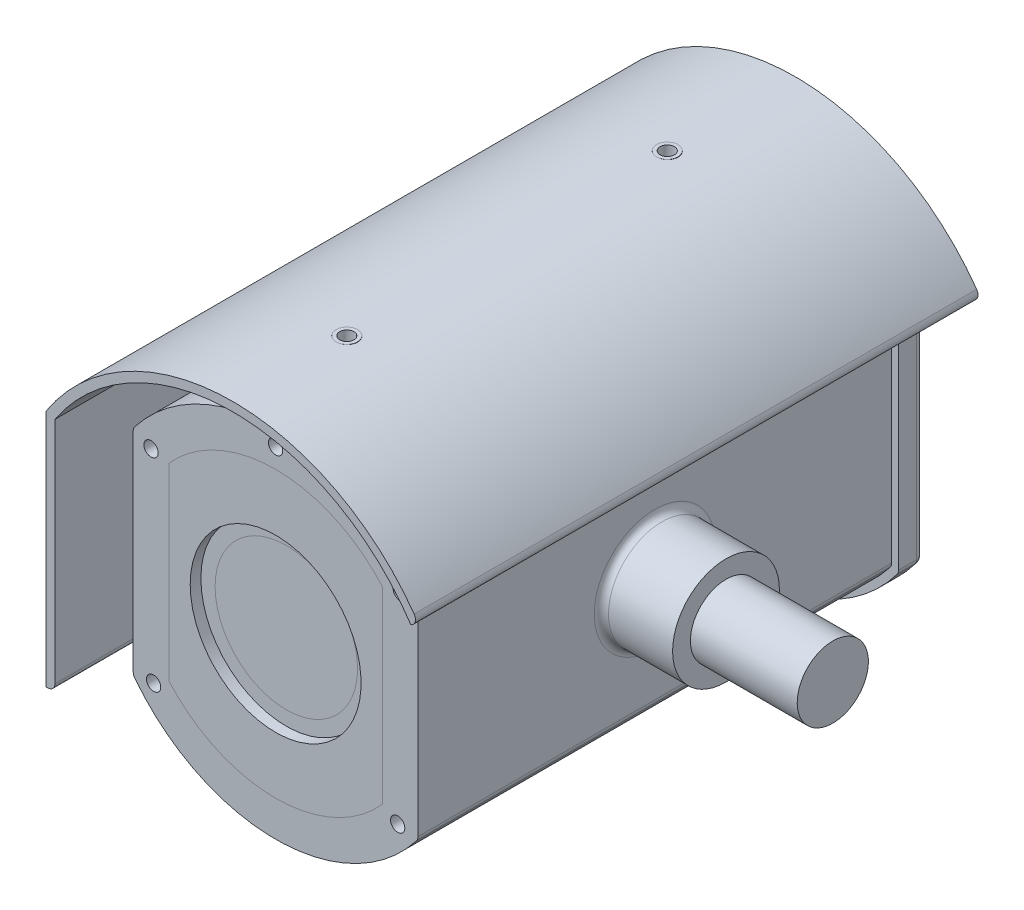
from build123d import *

# Parameters (mm, degrees)
BOSS_EXTRUDE1_DEPTH      = 140
CUT_EXTRUDE1_DEPTH       = 7
BOSS_EXTRUDE2_DEPTH      = 12
BOSS_EXTRUDE2_DEPTH_BACK = 146
SKETCH4_R                = 24
SKETCH4_R_2              = 20
BOSS_EXTRUDE3_DEPTH      = 4
CUT_EXTRUDE2_START       = -7
SKETCH5_R                = 20
CUT_EXTRUDE2_DEPTH       = 7
SKETCH6_R                = 11
CUT_EXTRUDE3_DEPTH       = 1
DOME1_FACE_RADIUS        = 11
DOME1_HEIGHT             = 5
SKETCH7_R                = 3
BOSS_EXTRUDE4_DEPTH      = 12.5
SKETCH8_R                = 2
CUT_EXTRUDE4_DEPTH       = 17
BOSS_EXTRUDE5_REACH      = 198.256
BOSS_EXTRUDE5_END_RADIUS = 50
SKETCH9_R                = 3
SKETCH10_R               = 2
CUT_EXTRUDE5_DEPTH       = 17
BOSS_EXTRUDE6_DEPTH      = 7
SKETCH12_W               = 70
SKETCH12_H               = 3.5
CUT_EXTRUDE6_DEPTH       = 5
SKETCH14_R               = 20
BOSS_EXTRUDE7_DEPTH      = 2
SKETCH15_R               = 24
BOSS_EXTRUDE8_DEPTH      = 5
SKETCH16_R               = 2
CUT_EXTRUDE8_DEPTH       = 5
CUT_EXTRUDE7_DEPTH       = 303.977741111
CUT_EXTRUDE7_DEPTH_BACK  = 303.977741111
SKETCH13_R               = 124.287084565
SKETCH17_R               = 10
BOSS_EXTRUDE9_DEPTH      = 50
SKETCH18_R               = 15
SKETCH18_R_2             = 10
BOSS_EXTRUDE10_DEPTH     = 20
FILLET1_R                = 2
SCALE1_SCALE             = 0.5


with BuildPart() as part:
    # Sketch1 → Boss-Extrude1 (new body)
    with BuildSketch(Plane.XY):
        with BuildLine():
            Line((-40, -30), (-40, 30))
            ThreePointArc((-40, 30), (0, 50), (40, 30))
            Line((40, 30), (40, -30))
            ThreePointArc((40, -30), (0, -50), (-40, -30))
        make_face()
    extrude(amount=BOSS_EXTRUDE1_DEPTH)

    # Sketch2 → Cut-Extrude1 (cut)
    with BuildSketch(Plane.XY.offset(140)):
        with BuildLine():
            Line((-30, 26.457513111), (-30, -26.457513111))
            ThreePointArc((-30, -26.457513111), (0, -40), (30, -26.457513111))
            Line((30, -26.457513111), (30, 26.457513111))
            ThreePointArc((30, 26.457513111), (0, 40), (-30, 26.457513111))
        make_face()
    extrude(amount=-CUT_EXTRUDE1_DEPTH, mode=Mode.SUBTRACT)

    # Sketch4 → Boss-Extrude3 (add)
    with BuildSketch(Plane.XY.offset(133)):
        Circle(SKETCH4_R)
        Circle(SKETCH4_R_2, mode=Mode.SUBTRACT)
    extrude(amount=BOSS_EXTRUDE3_DEPTH)

    # Sketch5 → Cut-Extrude2 (cut)
    with BuildSketch(Plane.XY.offset(133).offset(CUT_EXTRUDE2_START)):
        Circle(SKETCH5_R)
    extrude(amount=CUT_EXTRUDE2_DEPTH, mode=Mode.SUBTRACT)

    # Sketch6 → Cut-Extrude3 (cut)
    with BuildSketch(Plane.XY.offset(126)):
        Circle(SKETCH6_R)
    extrude(amount=-CUT_EXTRUDE3_DEPTH, mode=Mode.SUBTRACT)

    # Dome1: a dome of height H over a round flat face of radius A is a cap of a sphere of radius (A * A + H * H) / (2 * H)
    dome1_r = (DOME1_FACE_RADIUS * DOME1_FACE_RADIUS + DOME1_HEIGHT * DOME1_HEIGHT) / (2 * DOME1_HEIGHT)
    dome1_base = Plane((0, 0, 125), z_dir=(0, 0, 1))
    with Locations(dome1_base.offset(DOME1_HEIGHT - dome1_r)):
        dome1_ball = Sphere(dome1_r, mode=Mode.PRIVATE)
    add(split(dome1_ball, bisect_by=dome1_base, keep=Keep.TOP, mode=Mode.PRIVATE))



with BuildPart() as body_2:
    # Sketch3 → Boss-Extrude2 (new, two sides: drawn at the far end of the back side and taken through both)
    with BuildSketch(Plane.XY.offset(140).offset(-BOSS_EXTRUDE2_DEPTH_BACK)):
        with BuildLine():
            Line((52.5, -33.166247904), (52.5, 33.911649916))
            ThreePointArc((52.5, 33.911649916), (0.380386371, 62.498842439), (-52.083333333, 34.5481749))
            Line((-52.083333333, 34.5481749), (-50, 33.166247904))
            ThreePointArc((-50, 33.166247904), (0, 60), (50, 33.166247904))
            Line((50, 33.166247904), (50, -33.166247904))
            Line((50, -33.166247904), (52.5, -33.166247904))
        make_face()
    extrude(amount=BOSS_EXTRUDE2_DEPTH + BOSS_EXTRUDE2_DEPTH_BACK)


with BuildPart() as part_1:
    add(part.part)

    add(body_2.part)  # Boss-Extrude4 merges body 2
    # Sketch7 → Boss-Extrude4 (add)
    with BuildSketch(Plane(origin=(52.5, 0, 0), x_dir=(0, 0, -1), z_dir=(1, 0, 0))):
        with Locations(Location((-120, 0, 0), (0, 0, 270))):
            Circle(SKETCH7_R)
        with Locations(Location((-30, 0, 0), (0, 0, 270))):
            Circle(SKETCH7_R)
    extrude(amount=-BOSS_EXTRUDE4_DEPTH)

    # Sketch8 → Cut-Extrude4 (cut)
    with BuildSketch(Plane(origin=(52.5, 0, 0), x_dir=(0, 0, -1), z_dir=(1, 0, 0))):
        with Locations((-120, 0)):
            Circle(SKETCH8_R)
        with Locations((-30, 0)):
            Circle(SKETCH8_R)
    extrude(amount=-CUT_EXTRUDE4_DEPTH, mode=Mode.SUBTRACT)

    # Boss-Extrude5: up to this cylinder (the profile starts outside it)
    boss_extrude5_end = Plane(origin=(0, 0, 75), z_dir=(0, 0, -1)) * Cylinder(BOSS_EXTRUDE5_END_RADIUS, 587.512, mode=Mode.PRIVATE)
    # Sketch9 → Boss-Extrude5 (add, up to the surface)
    with BuildSketch(Plane(origin=(0, 62.5, 0), x_dir=(-1, 0, 0), z_dir=(0, 1, 0)), mode=Mode.PRIVATE) as boss_extrude5_sk1:
        with Locations(Location((0, 120, 0), (0, 0, 90))):
            Circle(SKETCH9_R)
    boss_extrude5_tool1 = extrude(boss_extrude5_sk1.sketch, amount=-BOSS_EXTRUDE5_REACH, mode=Mode.PRIVATE) - boss_extrude5_end
    add(boss_extrude5_tool1.solids().sort_by_distance((0, 62.5, 120))[0])
    # Sketch9 → Boss-Extrude5 (add, up to the surface)
    with BuildSketch(Plane(origin=(0, 62.5, 0), x_dir=(-1, 0, 0), z_dir=(0, 1, 0)), mode=Mode.PRIVATE) as boss_extrude5_sk2:
        with Locations(Location((0, 30, 0), (0, 0, 90))):
            Circle(SKETCH9_R)
    boss_extrude5_tool2 = extrude(boss_extrude5_sk2.sketch, amount=-BOSS_EXTRUDE5_REACH, mode=Mode.PRIVATE) - boss_extrude5_end
    add(boss_extrude5_tool2.solids().sort_by_distance((0, 62.5, 30))[0])

    # Sketch10 → Cut-Extrude5 (cut)
    with BuildSketch(Plane(origin=(0, 62.5, 0), x_dir=(1, 0, 0), z_dir=(0, 1, 0))):
        with Locations(Location((0, -30, 0), (0, 0, 270))):
            Circle(SKETCH10_R)
        with Locations(Location((0, -120, 0), (0, 0, 270))):
            Circle(SKETCH10_R)
    extrude(amount=-CUT_EXTRUDE5_DEPTH, mode=Mode.SUBTRACT)

    # Sketch11 → Boss-Extrude6 (add)
    with BuildSketch(Plane(origin=(0, 0, 0), x_dir=(-1, 0, 0), z_dir=(0, 0, -1))):
        with BuildLine():
            Line((-42, 30.659419434), (-42, -30.659419434))
            ThreePointArc((-42, -30.659419434), (0, -52), (42, -30.659419434))
            Line((42, -30.659419434), (42, 30.659419434))
            ThreePointArc((42, 30.659419434), (0, 52), (-42, 30.659419434))
        make_face()
        with BuildLine():
            Line((-40, 30), (-40, -30))
            ThreePointArc((-40, -30), (0, -50), (40, -30))
            Line((40, -30), (40, 30))
            ThreePointArc((40, 30), (0, 50), (-40, 30))
        make_face(mode=Mode.SUBTRACT)
    extrude(amount=-BOSS_EXTRUDE6_DEPTH)

    # Sketch12 → Cut-Extrude6 (cut)
    with BuildSketch(Plane(origin=(0, 0, 0), x_dir=(-1, 0, 0), z_dir=(0, 0, -1))):
        with BuildLine():
            ThreePointArc((16.155494421, 42), (0, 45), (-16.155494421, 42))
            Line((-16.155494421, 42), (16.155494421, 42))
        make_face()
        with BuildLine():
            ThreePointArc((-21.558061137, 39.5), (-24.342017693, 37.84793488), (-27, 36))
            Line((-27, 36), (27, 36))
            ThreePointArc((27, 36), (24.342017693, 37.84793488), (21.558061137, 39.5))
            Line((21.558061137, 39.5), (-21.558061137, 39.5))
        make_face()
        with BuildLine():
            ThreePointArc((-30.045798375, 33.5), (-31.841535092, 31.798060365), (-33.541019662, 30))
            Line((-33.541019662, 30), (33.541019662, 30))
            ThreePointArc((33.541019662, 30), (31.841535092, 31.798060365), (30.045798375, 33.5))
            Line((30.045798375, 33.5), (-30.045798375, 33.5))
        make_face()
        with Locations((0, 25.75)):
            Rectangle(SKETCH12_W, SKETCH12_H)
        with Locations((0, 19.75)):
            Rectangle(SKETCH12_W, SKETCH12_H)
        with Locations((0, 13.75)):
            Rectangle(SKETCH12_W, SKETCH12_H)
        with Locations((0, 7.75)):
            Rectangle(SKETCH12_W, SKETCH12_H)
        with Locations((0, 1.75)):
            Rectangle(SKETCH12_W, SKETCH12_H)
        with Locations((0, -4.25)):
            Rectangle(SKETCH12_W, SKETCH12_H)
        with Locations((0, -10.25)):
            Rectangle(SKETCH12_W, SKETCH12_H)
        with Locations((0, -16.25)):
            Rectangle(SKETCH12_W, SKETCH12_H)
        with Locations((0, -22.25)):
            Rectangle(SKETCH12_W, SKETCH12_H)
        with BuildLine():
            Line((35, -26.5), (-35, -26.5))
            Line((-35, -26.5), (-35, -28.284271247))
            ThreePointArc((-35, -28.284271247), (-34.281245243, -29.151264546), (-33.541019662, -30))
            Line((-33.541019662, -30), (33.541019662, -30))
            ThreePointArc((33.541019662, -30), (34.281245243, -29.151264546), (35, -28.284271247))
            Line((35, -28.284271247), (35, -26.5))
        make_face()
        with BuildLine():
            Line((31.124748995, -32.5), (-31.124748995, -32.5))
            ThreePointArc((-31.124748995, -32.5), (-29.115015223, -34.31203708), (-27, -36))
            Line((-27, -36), (27, -36))
            ThreePointArc((27, -36), (29.115015223, -34.31203708), (31.124748995, -32.5))
        make_face()
        with BuildLine():
            Line((23.296995514, -38.5), (-23.296995514, -38.5))
            ThreePointArc((-23.296995514, -38.5), (-19.803717846, -40.408077899), (-16.155494421, -42))
            Line((-16.155494421, -42), (16.155494421, -42))
            ThreePointArc((16.155494421, -42), (19.803717846, -40.408077899), (23.296995514, -38.5))
        make_face()
    extrude(amount=-CUT_EXTRUDE6_DEPTH, mode=Mode.SUBTRACT)

    # Sketch16 → Cut-Extrude8 (cut)
    with BuildSketch(Plane.XY.offset(140)):
        with Locations((35, 27.5)):
            Circle(SKETCH16_R)
        with Locations((-35, 27.5)):
            Circle(SKETCH16_R)
        with Locations((0, 45.5)):
            Circle(SKETCH16_R)
        with Locations((34.281245243, -29.151264546)):
            Circle(SKETCH16_R)
        with Locations((-34.281245243, -29.151264546)):
            Circle(SKETCH16_R)
    extrude(amount=-CUT_EXTRUDE8_DEPTH, mode=Mode.SUBTRACT)


with BuildPart() as body_2_2:
    # Sketch14 → Boss-Extrude7 (new body)
    with BuildSketch(Plane.XY.offset(137)):
        Circle(SKETCH14_R)
    extrude(amount=-BOSS_EXTRUDE7_DEPTH)


with BuildPart() as body_3:
    # Sketch15 → Boss-Extrude8 (new body)
    with BuildSketch(Plane.XY.offset(140)):
        with BuildLine():
            Line((-30, 26.457513111), (-30, -26.457513111))
            ThreePointArc((-30, -26.457513111), (0, -40), (30, -26.457513111))
            Line((30, -26.457513111), (30, 26.457513111))
            ThreePointArc((30, 26.457513111), (0, 40), (-30, 26.457513111))
        make_face()
        Circle(SKETCH15_R, mode=Mode.SUBTRACT)
    extrude(amount=-BOSS_EXTRUDE8_DEPTH)


with BuildPart() as body_4:
    # Mirror2: mirrored copy
    add(body_3.part.mirror(Plane(origin=(-101.014745231, 0, 0), x_dir=(0, 0, 1), z_dir=(1, 0, 0))))


with BuildPart() as body_5:
    # Mirror2 2: mirrored copy
    add(body_2_2.part.mirror(Plane(origin=(-101.014745231, 0, 0), x_dir=(0, 0, 1), z_dir=(1, 0, 0))))


with BuildPart() as body_6:
    # Mirror2 3: mirrored copy
    add(part_1.part.mirror(Plane(origin=(-101.014745231, 0, 0), x_dir=(0, 0, 1), z_dir=(1, 0, 0))))

    # Sketch17 → Boss-Extrude9 (add)
    with BuildSketch(Plane(origin=(-162.029490461, 0, 0), x_dir=(0, 0, -1), z_dir=(1, 0, 0))):
        with Locations(Location((-73.5, 0, 0), (0, 0, 270))):
            Circle(SKETCH17_R)
    extrude(amount=BOSS_EXTRUDE9_DEPTH)

    # Sketch18 → Boss-Extrude10 (add)
    with BuildSketch(Plane(origin=(-162.029490461, 0, 0), x_dir=(0, 0, -1), z_dir=(1, 0, 0))):
        with Locations(Location((-73.5, 0, 0), (0, 0, 270))):
            Circle(SKETCH18_R)
        with Locations(Location((-73.5, 0, 0), (0, 0, 90))):
            Circle(SKETCH18_R_2, mode=Mode.SUBTRACT)
    extrude(amount=BOSS_EXTRUDE10_DEPTH)

    # Fillet1
    fillet1_edges = [body_6.edges().sort_by_distance(p)[0] for p in [
        (-244.029490461, 30.659419434, 3.5),
        (-160.029490461, 30.659419434, 3.5),
        (-160.029490461, -30.659419434, 3.5),
        (-244.029490461, -30.659419434, 3.5),
        (-252.029490461, -33.166247904, 73),
        (-202.029490461, 52, 0),
        (-244.029490461, 0, 0),
        (-202.029490461, -52, 0),
        (-160.029490461, 0, 0),
        (-149.946157128, 34.5481749, 73),
        (-252.029490461, 3, 120),
        (-242.029490461, 3, 120),
        (-242.029490461, 30, 73.5),
        (-162.029490461, 30, 73.5),
        (-162.029490461, -30, 73.5),
        (-242.029490461, -30, 73.5),
        (-162.029490461, 15, 73.5),
        (-252.029490461, 3, 30),
        (-242.029490461, 3, 30),
        (-202.029490459, 60.000000006, 117.000000018),
        (-202.029490459, 50.000000007, 117.000000018),
        (-202.029490461, 59.999999997, 26.999999988),
        (-202.029490461, 49.999999997, 26.999999988),
    ]]
    fillet(fillet1_edges, radius=FILLET1_R)


with BuildPart() as cut_extrude7_tool:
    # Sketch13 → Cut-Extrude7 (new, two sides: drawn at the far end of the back side and taken through both)
    with BuildSketch(Plane.XY.offset(-CUT_EXTRUDE7_DEPTH_BACK)):
        Circle(SKETCH13_R)
    extrude(amount=CUT_EXTRUDE7_DEPTH + CUT_EXTRUDE7_DEPTH_BACK)


with BuildPart() as part_2:
    add(part_1.part)

    # Cut-Extrude7: cut by cut_extrude7_tool
    add(cut_extrude7_tool.part, mode=Mode.SUBTRACT)


with BuildPart() as body_2_2_1:
    add(body_2_2.part)

    # Cut-Extrude7: cut by cut_extrude7_tool
    add(cut_extrude7_tool.part, mode=Mode.SUBTRACT)


with BuildPart() as body_3_1:
    add(body_3.part)

    # Cut-Extrude7: cut by cut_extrude7_tool
    add(cut_extrude7_tool.part, mode=Mode.SUBTRACT)


with BuildPart() as body_6_1:
    # Scale1: scaled about (0, 0, 0)
    add(body_6.part.scale(SCALE1_SCALE))


with BuildPart() as body_4_1:
    # Scale1: scaled about (0, 0, 0)
    add(body_4.part.scale(SCALE1_SCALE))


with BuildPart() as body_5_1:
    # Scale1: scaled about (0, 0, 0)
    add(body_5.part.scale(SCALE1_SCALE))


solid = Compound([body_6_1.part, body_4_1.part, body_5_1.part])
